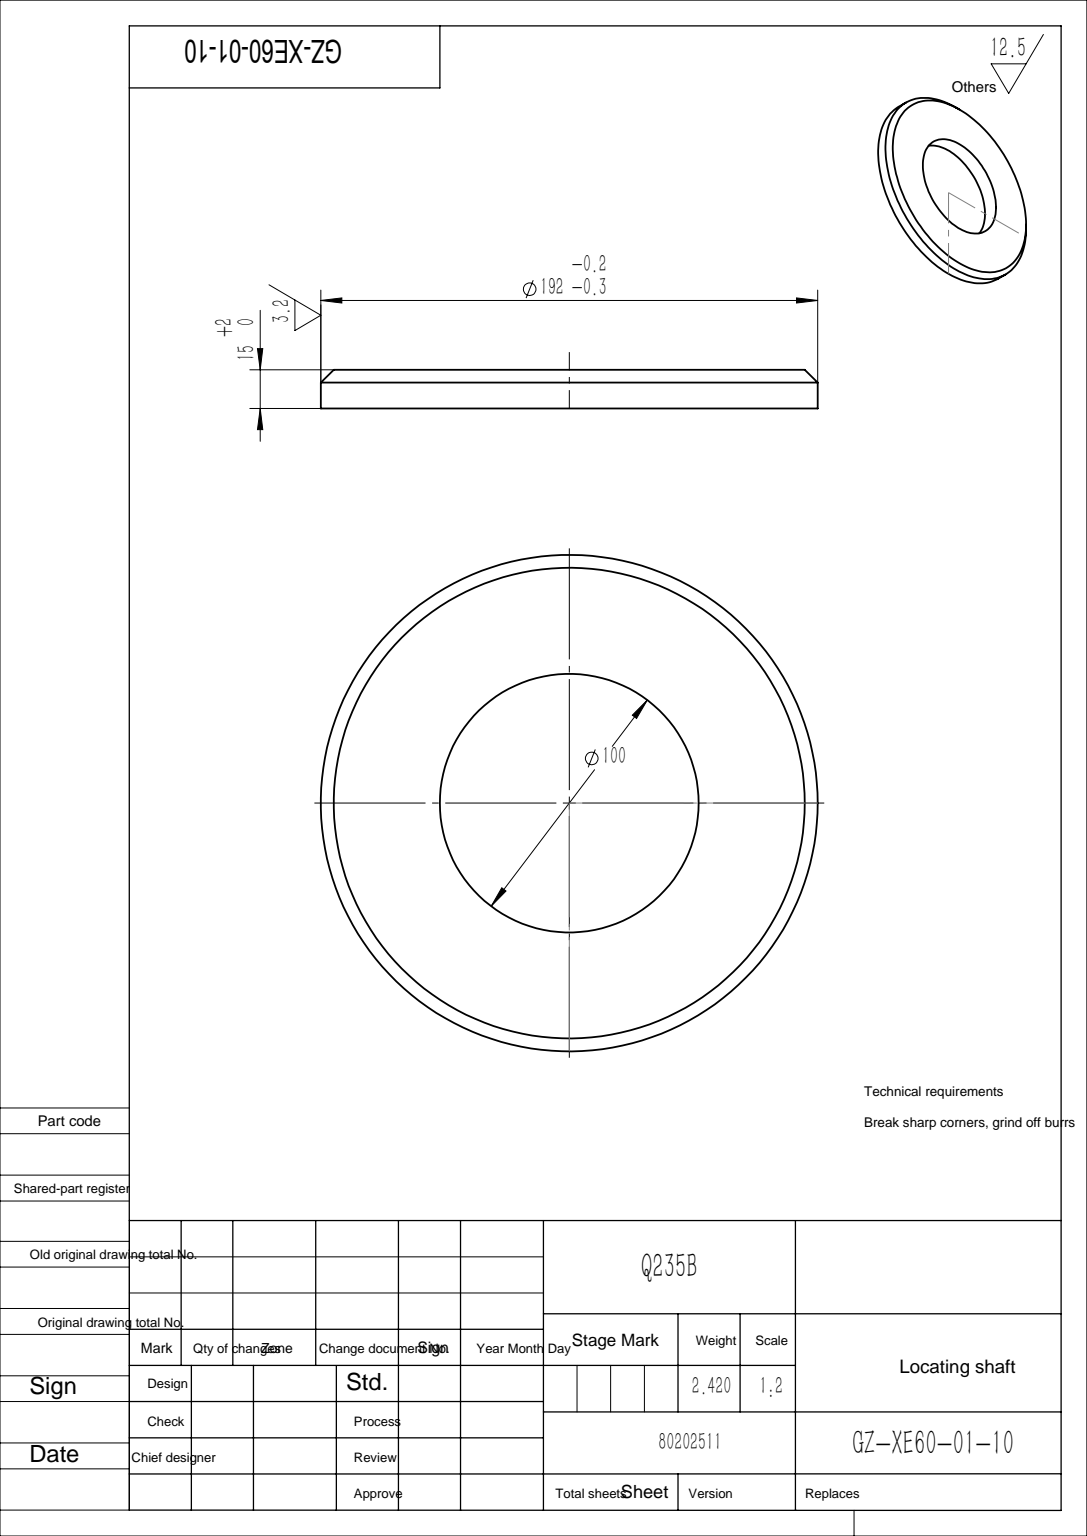
from build123d import *

# Parameters (mm, degrees)
SKETCH1_R           = 96
SKETCH1_R_2         = 50
BOSS_EXTRUDE1_DEPTH = 15
CHAMFER1_SIZE       = 5


with BuildPart() as part:
    # Sketch1 → Boss-Extrude1 (new body)
    with BuildSketch(Plane.XY):
        Circle(SKETCH1_R)
        Circle(SKETCH1_R_2, mode=Mode.SUBTRACT)
    extrude(amount=BOSS_EXTRUDE1_DEPTH)

    # Chamfer1
    chamfer1_edges = [part.edges().sort_by_distance(p)[0] for p in [
        (-96, 0, 15),
    ]]
    chamfer(chamfer1_edges, length=CHAMFER1_SIZE)


solid = part.part
